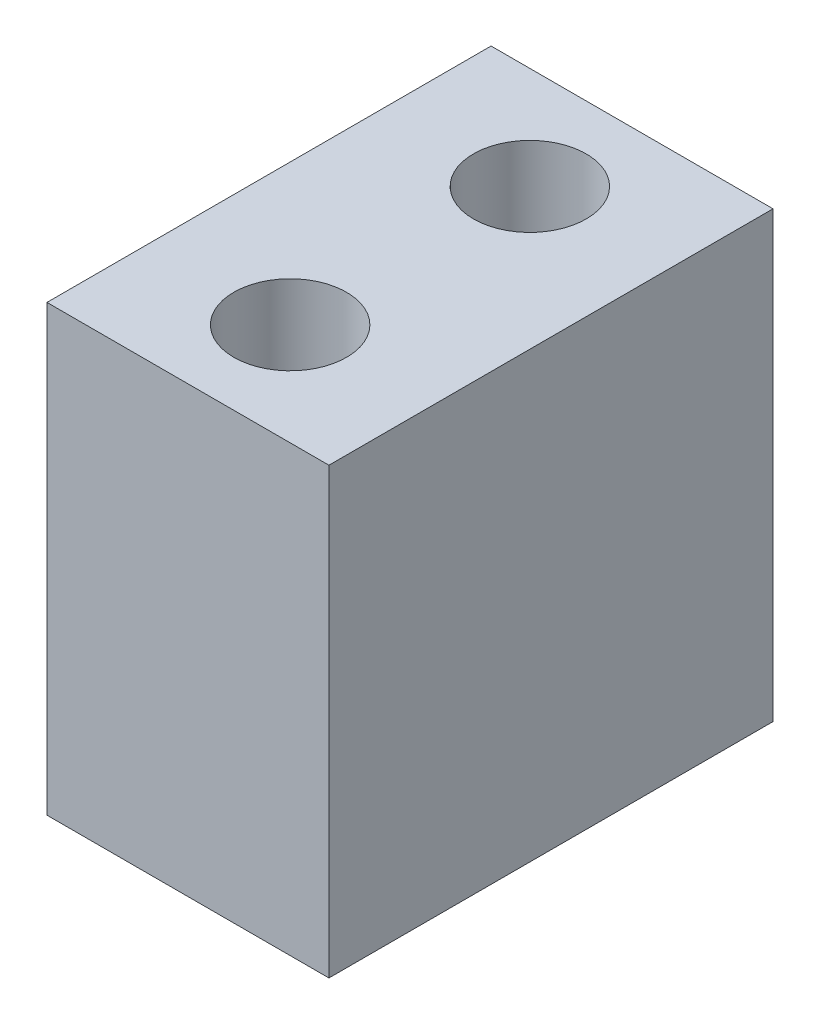
from build123d import *

# Parameters (mm, degrees)
SKETCH2_W              = 80
SKETCH2_H              = 126
BOSS_EXTRUDE1_DEPTH    = 63
M36_TAPPED_HOLE1_D     = 32
M36_TAPPED_HOLE1_DEPTH = 80
M36_TAPPED_HOLE1_TIP   = 9.613769904


with BuildPart() as part:
    # Sketch2 → Boss-Extrude1 (new, symmetric)
    with BuildSketch(Plane(origin=(0, 0, 0), x_dir=(1, 0, 0), z_dir=(0, 1, 0))):
        Rectangle(SKETCH2_W, SKETCH2_H)
    extrude(amount=BOSS_EXTRUDE1_DEPTH, both=True)

    # M36 Tapped Hole1
    with Locations(Plane(origin=(0, 63, 0), x_dir=(1, 0, 0), z_dir=(0, 1, 0))):
        with Locations((0, 34), (0, -34)):
            Hole(M36_TAPPED_HOLE1_D / 2, depth=M36_TAPPED_HOLE1_DEPTH)
            with Locations((0, 0, -(M36_TAPPED_HOLE1_DEPTH + M36_TAPPED_HOLE1_TIP / 2))):  # 118° drill point
                Cone(0, M36_TAPPED_HOLE1_D / 2, M36_TAPPED_HOLE1_TIP, mode=Mode.SUBTRACT)


solid = part.part
